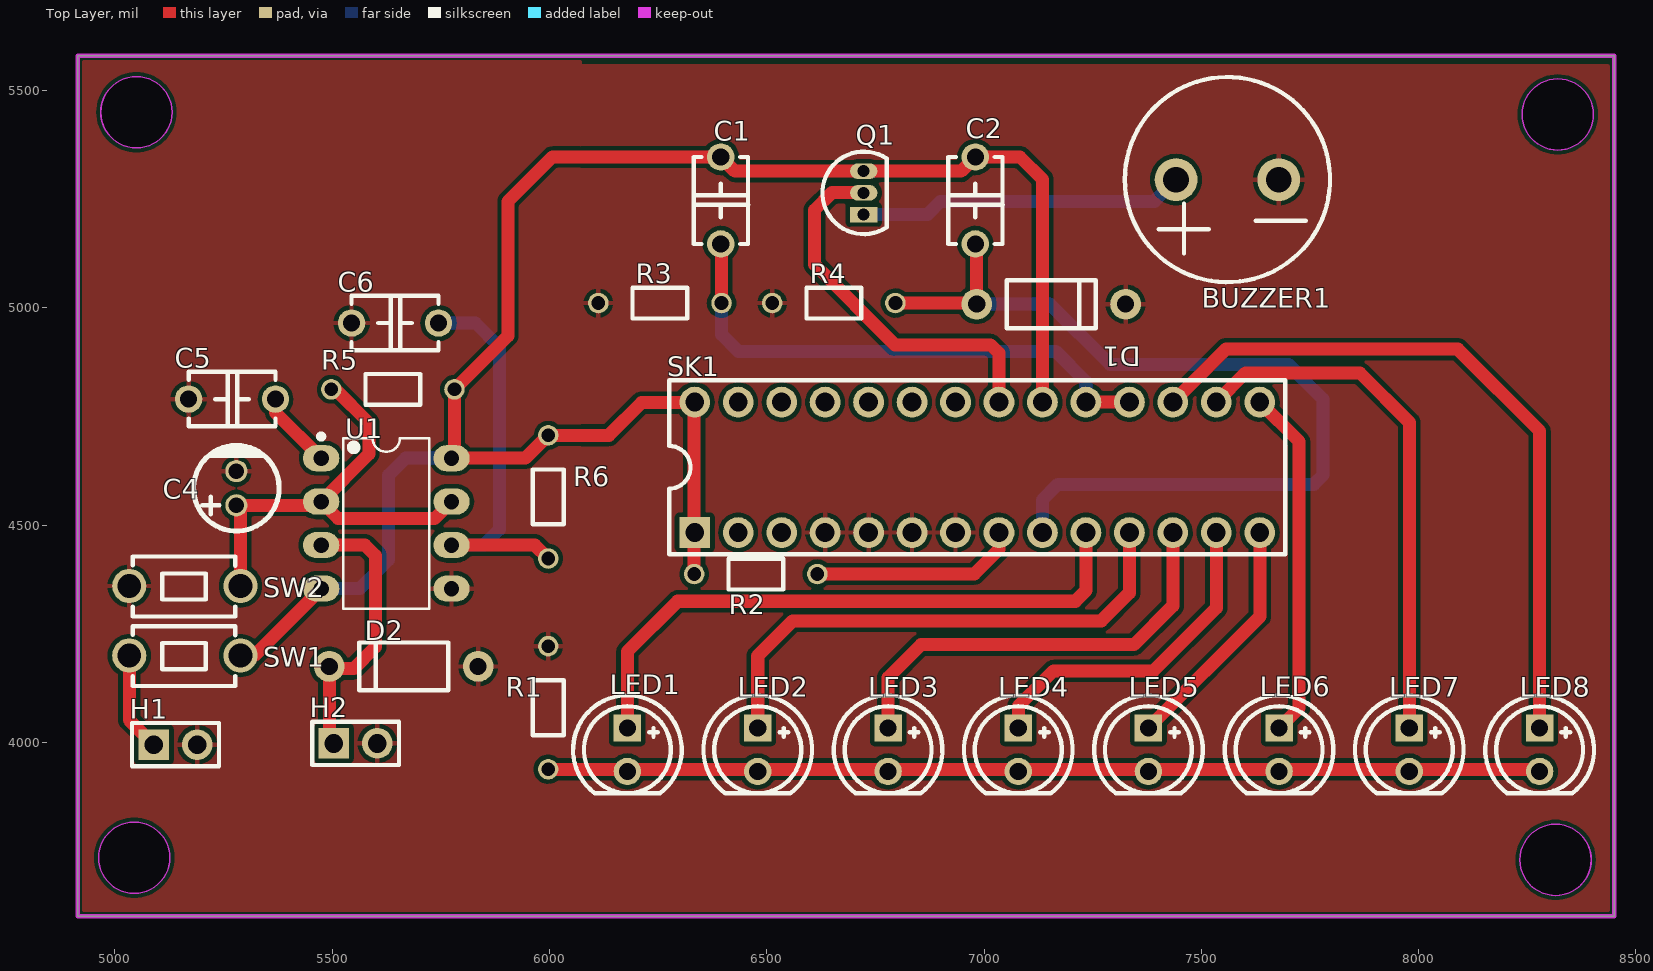
[diagram p0: Top Layer view]
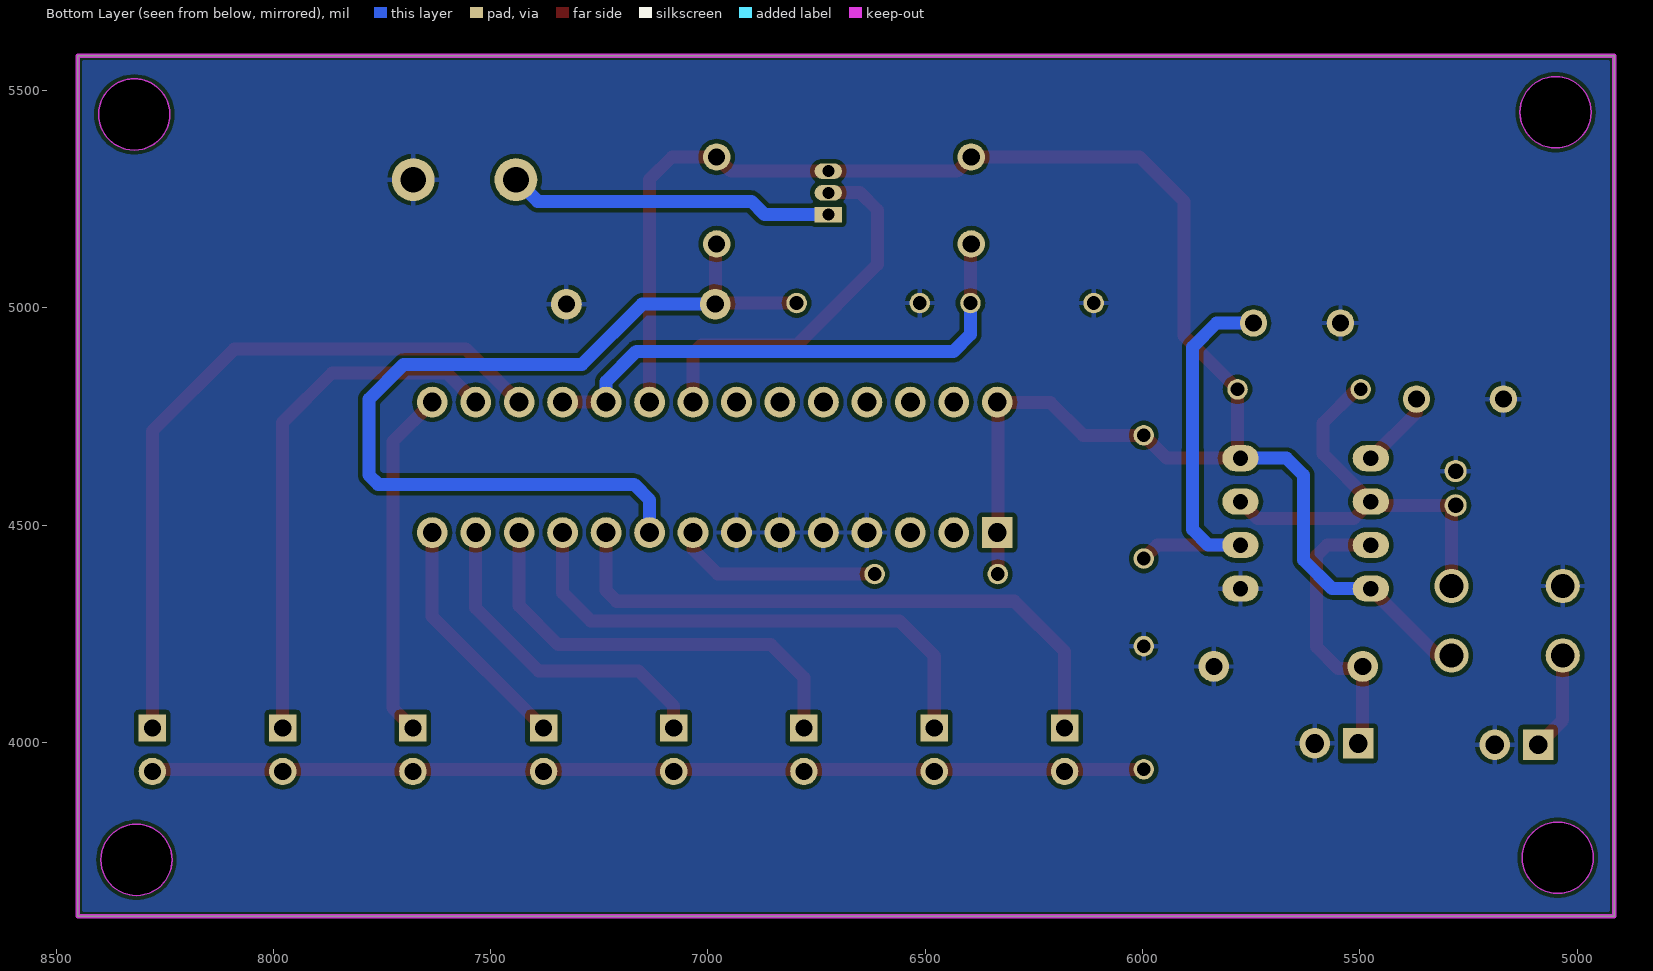
[diagram p1: Bottom Layer view, seen from below]
# Altium PCB MISC75112.pcbdoc
Units mil, origin at the board's own origin, x right, y up, seen from the top; angles counter-clockwise.
Board outline 3535 x 1980 mil, 2 copper layers (Top Layer, Bottom Layer), stack 62.206 mil thick; 29 components, 21 nets, 91 pads, 0 vias.

## Layer stack, top to bottom
Top Solder Mask Layer: solder mask 0.394, Dk 3.3
Top Layer: signal copper 1.379
Dielectric1: surface 59.449, FR4, Dk 4.5
Bottom Layer: signal copper 1.378
Bottom Solder Mask Layer: solder mask 0.394, Dk 3.3

## Board outline
4915,5580 4915,3600 8450,3600 8450,5580
cut-out: 5132.01,5450 cw(c5050,5450) 4967.99,5450 cw(c5050,5450)
cut-out: 8402.01,5445 cw(c8320,5445) 8237.99,5445 cw(c8320,5445)
cut-out: 8397.01,3730 cw(c8315,3730) 8232.99,3730 cw(c8315,3730)
cut-out: 5127.01,3735 cw(c5045,3735) 4962.99,3735 cw(c5045,3735)

## Design rules (kind name [scope] priority, off if disabled: settings)
BoardOutlineClearance copperThickness2oz_1 [All] p2 off: genericclearance=7.99 ignorepadtopadclearanceinfootprint=FALSE except(0: Arc-SplitContinuation Track-SplitContinuation SMDPad-SplitContinuation THPad-SplitContinuation Via-SplitContinuation Fill-SplitContinuation Region-SplitContinuation Poly-SplitContinuation Text-SplitContinuation Hole-SplitContinuation; 5.98: Arc-CutoutEdge SMDPad-CutoutEdge THPad-CutoutEdge Via-CutoutEdge Fill-CutoutEdge Region-CutoutEdge Text-CutoutEdge; 6.93: Hole-OutlineEdge Hole-CutoutEdge; 10: Poly-OutlineEdge Poly-CutoutEdge; 11.81: Arc-OutlineEdge Track-OutlineEdge SMDPad-OutlineEdge THPad-OutlineEdge Via-OutlineEdge Fill-OutlineEdge Region-OutlineEdge Text-OutlineEdge Track-CutoutEdge)
BoardOutlineClearance copperThickness1oz_1 [All] p4: genericclearance=4.02 ignorepadtopadclearanceinfootprint=FALSE except(0: Arc-SplitContinuation Track-SplitContinuation SMDPad-SplitContinuation THPad-SplitContinuation Via-SplitContinuation Fill-SplitContinuation Region-SplitContinuation Poly-SplitContinuation Text-SplitContinuation Hole-SplitContinuation; 6: SMDPad-CutoutEdge THPad-CutoutEdge Via-CutoutEdge Fill-CutoutEdge Region-CutoutEdge Text-CutoutEdge; 6.93: Hole-OutlineEdge Hole-CutoutEdge; 10: Poly-OutlineEdge Poly-CutoutEdge; 11.8: Arc-OutlineEdge Track-OutlineEdge SMDPad-OutlineEdge THPad-OutlineEdge Via-OutlineEdge Fill-OutlineEdge Region-OutlineEdge Text-OutlineEdge; 11.81: Arc-CutoutEdge Track-CutoutEdge)
Clearance copperThickness2oz [All] p1 off: gap=7.99 ignorepadtopadclearanceinfootprint=FALSE except(5.98: SMDPad-Track SMDPad-SMDPad THPad-Track SMDPad-THPad THPad-THPad Track-Via SMDPad-Via THPad-Via Via-Via Fill-Track Region-Track Fill-SMDPad Region-SMDPad Fill-THPad Region-THPad Fill-Via Region-Via Fill-Fill Fill-Region Region-Region Arc-Track Arc-SMDPad Arc-THPad Arc-Via Fill-Arc Region-Arc Arc-Arc Text-Track SMDPad-Text Text-THPad Text-Via Fill-Text Region-Text Arc-Text Text-Text; 6.93: Hole-Track Hole-SMDPad Hole-THPad Hole-Via Fill-Hole Region-Hole Hole-Arc Hole-Text; 10: Poly-Track Poly-SMDPad Poly-THPad Poly-Via Poly-Fill Poly-Region Poly-Poly Poly-Arc Poly-Text Poly-Hole)
Clearance copperThickness1oz [All] p3: gap=4.02 ignorepadtopadclearanceinfootprint=FALSE except(5.98: SMDPad-Track SMDPad-SMDPad THPad-Track SMDPad-THPad THPad-THPad Track-Via SMDPad-Via THPad-Via Via-Via Fill-Track Region-Track Fill-SMDPad Region-SMDPad Fill-THPad Region-THPad Fill-Via Region-Via Fill-Fill Fill-Region Region-Region; 6: Arc-Track Arc-SMDPad Arc-THPad Arc-Via Fill-Arc Region-Arc Arc-Arc Text-Track SMDPad-Text Text-THPad Text-Via Fill-Text Region-Text Arc-Text Text-Text; 6.93: Hole-Track Hole-SMDPad Hole-THPad Hole-Via Fill-Hole Region-Hole Hole-Arc Hole-Text; 10: Poly-Track Poly-SMDPad Poly-THPad Poly-Via Poly-Fill Poly-Region Poly-Poly Poly-Arc Poly-Text Poly-Hole)
Creepage creepage [All] p1: checkdistance=0 ignoreinternallayers=TRUE applytopolygonpour=TRUE
DiffPairsRouting differentialPair [All] p1: maxlimit=6 minlimit=6 mostfreqgap=6 toplayer_minwidth=5 toplayer_prefwidth=10 toplayer_maxwidth=100 toplayer_mingap=6 toplayer_prefgap=6 toplayer_maxgap=6 bottomlayer_minwidth=5 bottomlayer_prefwidth=10 bottomlayer_maxwidth=100 bottomlayer_mingap=6 bottomlayer_prefgap=6 bottomlayer_maxgap=6 maxuncoupledlength=10
HoleToHoleClearance otherClearance [All] p1: gap=11.81 allowstackedmicrovias=TRUE
Length netLength [All] p1: minlimit=0 maxlimit=0
MatchedLengths netLengthTolerance [All] p1: tolerance=1000
PasteMaskExpansion pasteMaskExpansion [All] p1: expansion=0
PlaneConnect innerPlane [All] p1: planeconnectstyle=Relief reliefexpansion=20 reliefentries=4 reliefconductorwidth=10 reliefairgap=10
PolygonConnect copperRegion [(InNet('GND'))] p1: connectstyle=Relief reliefconductorwidth=10 reliefentries=4 polygonreliefangle="90 Angle" airgapwidth=10 via.connectstyle=Relief via.reliefconductorwidth=10 via.reliefentries=4 via.polygonreliefangle="90 Angle" via.airgapwidth=10
RoutingVias viaSize [All] p1: holewidth=12.01 width=24.02 viastyle="Through Hole" minholewidth=11.81 minwidth=19.68 maxholewidth=248.03 maxwidth=393.7
SolderMaskExpansion solderMaskExpansion [IsVia] p1: expansion=-1000 istentingtop=TRUE
SolderMaskExpansion solderMaskExpansion [All] p2: expansion=2 istentingtop=FALSE
Width copperThickness2oz_2 [All] p1 off: maxlimit=100 minlimit=8 preferedwidth=10
Width copperThickness1oz_2 [All] p2: maxlimit=100 minlimit=5 preferedwidth=10

## Components (designator, comment, footprint, x,y, rotation, side; value= is the part's Value field where it differs from the comment)
BUZZER1 "buzzer" BUZ-TH_BD12.0-P6.00-D0.9-RD 7560,5295 r180 top
C1 "0.1uF" CAP-TH_L5.1-W3.2-P5.08-D0.50 6394.47,5247.04 r90 top
C2 "0.047uF" CAP-TH_L5.1-W3.2-P5.08-D0.50 6980,5247.04 r90 top
C4 "10uF" CAP-TH_BD5.0-P2.00-D0.8-FD-10UF50VC110GL 5280,4585 r90 top
C5 "10nF" CAP-TH_L5.1-W3.2-P5.08-D0.50 5270,4790 r0 top
C6 "10nF" CAP-TH_L5.1-W3.2-P5.08-D0.50 5645,4965 r0 top
D1 "" DO_1N4007 7154.47,5008.49 r180 top
D2 "" DO_1N4007 5665,4175 r0 top
H1 "" HDR-TH_2P-P2.54-V-M-1 5140,3995 r0 top
H2 "" HDR-TH_2P-P2.54-V-M-1 5554.18,3998.07 r0 top
LED1 "" LED-TH_5mm 6179.47,3983.38 r270 top
LED2 "" LED-TH_5mm 6479.47,3983.38 r270 top
LED3 "" LED-TH_5mm 6779.47,3983.38 r270 top
LED4 "" LED-TH_5mm 7078.88,3983.38 r270 top
LED5 "" LED-TH_5mm 7378.29,3983.38 r270 top
LED6 "" LED-TH_5mm 7678.99,3983.38 r270 top
LED7 "" LED-TH_5mm 7978.4,3983.38 r270 top
LED8 "" LED-TH_5mm 8278.4,3983.38 r270 top
Q1 "" S8050_TO_92 6723.29,5264.53 r90 top
R1 "1kΩ" Res_1/8W 5995,4080 r270 top
R2 "22kΩ" Res_1/8W 6475,4390 r180 top
R3 "100kΩ" Res_1/8W 6254.47,5008.49 r0 top
R4 "100kΩ" Res_1/8W 6654.47,5008.49 r0 top
R5 "10kΩ" Res_1/8W 5640,4810 r0 top
R6 "10kΩ" Res_1/8W 6000,4565 r90 top
SK1 "X5621WV-2x14-C762D1000-1000" DIP-28_L35.6-W10.2-P2.54-LS7.6-BL 6984.47,4633.07 r0 top
SW1 "" Key_TH_3.5x6x4.3 5155,4200 r0 top
SW2 "" Key_TH_3.5x6x4.3 5155,4360 r0 top
U1 "NE555" DIP-8_L9.8-W6.4-P2.54-LS7.6-BL 5624.93,4504.05 r270 top

## Footprints (in the part's own frame and the unit in brackets; to place one, negate y for a bottom-side part, rotate by r counter-clockwise, add the part's x,y. Pads: shape width x height; smd on the part's side, far side on the other; paste and mask are expansions set on the pad)
BUZ-TH_BD12.0-P6.00-D0.9-RD [mm]
  round 2.5 hole 1.5 paste+0 mask+0.05: 1(-3,0) 2(3,0)
  silkscreen extent -5.99,-5.99 5.99,5.99
CAP-TH_BD5.0-P2.00-D0.8-FD-10UF50VC110GL [mm]
  round 1.3 hole 0.9 paste+0 mask+0.051: 1(-1,0) 2(1,0)
  silkscreen extent -2.5,-2.5 2.5,2.5
CAP-TH_L5.1-W3.2-P5.08-D0.50 [mm]
  round 1.6 hole 1 paste+0 mask+0.05: 1(-2.54,0) 2(2.54,0)
  silkscreen extent -2.54,-1.6 2.54,1.59
DIP-8_L9.8-W6.4-P2.54-LS7.6-BL [mil]
  oval 60x83.66 hole 35.43 paste+0 mask+2: 1(-150,-150) 2(-50,-150) 3(50,-150) 4(150,-150) 5(150,150) 6(50,150) 7(-50,150) 8(-150,150)
  silkscreen extent -206,-156 196,99
DIP-28_L35.6-W10.2-P2.54-LS7.6-BL [mm]
  rect 1.8x1.8 hole 1.1: 1(-16.51,-3.81)
  round 1.8 hole 1.1: 2(-13.97,-3.81) 3(-11.43,-3.81) 4(-8.89,-3.81) 5(-6.35,-3.81) 6(-3.81,-3.81) 7(-1.27,-3.81) 8(1.27,-3.81) 9(3.81,-3.81) 10(6.35,-3.81) 11(8.89,-3.81) 12(11.43,-3.81) 13(13.97,-3.81) 14(16.51,-3.81) 15(16.51,3.81) 16(13.97,3.81) 17(11.43,3.81) 18(8.89,3.81) 19(6.35,3.81) 20(3.81,3.81) 21(1.27,3.81) 22(-1.27,3.81) 23(-3.81,3.81) 24(-6.35,3.81) 25(-8.89,3.81) 26(-11.43,3.81) 27(-13.97,3.81) 28(-16.51,3.81)
  silkscreen extent -18,-5.08 18,5.08
DO_1N4007 [mm]
  round 1.8 hole 1 paste+0 mask+0.051: 1(-4.35,0) 2(4.35,0)
  silkscreen extent -2.6,-1.4 2.6,1.4
HDR-TH_2P-P2.54-V-M-1 [mm]
  rect 1.8x1.8 hole 1.1: 1(-1.27,0)
  round 1.8 hole 1.1: 2(1.27,0)
  silkscreen extent -2.54,-1.27 2.54,1.27
Key_TH_3.5x6x4.3 [mil]
  round 78.7 hole 55.1 paste+0 mask+2: A(-121.44,0) B(134.46,0)
  silkscreen extent -114,-70 123,68
LED-TH_5mm [mm]
  rect 1.6x1.6 hole 1 paste+0 mask+0.051: 1(-1.27,0)
  round 1.6 hole 1 paste+0 mask+0.051: 2(1.27,0)
  silkscreen extent -3.17,-3.17 2.54,3.17
Res_1/8W [mil]
  round 47.2 hole 31.5 paste+0 mask+2: 1(-141.7,2.48) 2(141.7,2.48)
  silkscreen extent -63,-33 63,38
S8050_TO_92 [mil]
  rect 35.4x63 hole 27.6 paste+0 mask+2: 1(-50,0)
  oval 35.4x63 hole 27.6 paste+0 mask+2: 2(0,0) 3(50,0)
  silkscreen extent -95,-53 95,95

## Nets (pads, with @x,y where several pads share a name; then routed paths per layer and width w, separated by ;. In a path a pad name is that pad's centre, name@x,y a point inside that pad or via, vN(x,y) a via of type N, cw(c..) or ccw(c..) an arc to the next point about the centre after c; other vN are vias at no path point)
$1N42: LED1.1 SK1.10 | length 1422.7
  Top Layer w30: LED1.1 6179.47,4209.47 6295,4325 7210,4325 7234.47,4349.47 SK1.10
$1N43: LED2.1 SK1.11 | length 1219.7
  Top Layer w30: LED2.1 6479.47,4199.47 6560,4280 7270,4280 7334.47,4344.47 SK1.11
$1N44: LED3.1 SK1.12 | length 1008
  Top Layer w30: LED3.1 6779.47,4149.47 6855,4225 7345,4225 7434.47,4314.47 SK1.12
$1N45: LED4.1 SK1.13 | length 773.1
  Top Layer w30: LED4.1 7078.88,4083.88 7160,4165 7390,4165 7534.47,4309.47 SK1.13
$1N46: LED5.1 SK1.14 | length 555.8
  Top Layer w30: LED5.1 7634.47,4289.56 SK1.14
$1N47: LED6.1 SK1.15 | length 806.2
  Top Layer w30: SK1.15 7725,4692.53 7725,4079.4 LED6.1
$1N48: LED7.1 SK1.16 | length 1221.8
  Top Layer w30: SK1.16 7601.4,4850 7865,4850 7978.4,4736.6 LED7.1
$1N49: LED8.1 SK1.17 | length 1655.7
  Top Layer w30: SK1.17 7556.4,4905 8090,4905 8278.4,4716.6 LED8.1
$1N50: LED1.2 LED2.2 LED3.2 LED4.2 LED5.2 LED6.2 LED7.2 LED8.2 R1.2 | length 2283
  Top Layer w30: R1.2 8273.48,3938.3 LED8.2
$1N52: C1.2 C2.2 Q1.3 R2.2 R5.2 R6.2 SK1.1 SK1.20 SK1.28 SW1.B U1.4 U1.8 | length 4272.4
  Top Layer w30: SW1.B 5320.88,4200 U1.4 ; R2.2 SK1.28@6333.3,4781.9 ; SK1.28 SK1.28@6333.3,4781.9 ; SK1.20 7134.47,5295.53 7082.96,5347.04 C2.2 6947.49,5314.53 Q1.3 6426.97,5314.53 C1.2 6007.04,5347.04 5905,5245 5905,4935.78 R5.2 5781.7,4660.82 U1.8 5944.88,4654.05 R6.2 6136.7,4706.7 6211.9,4781.9 SK1.28@6333.3,4781.9
  Bottom Layer w30: U1.4 5564.05,4354.05 5630,4420 5630,4615 5669.05,4654.05 U1.8
$1N53: R2.1 SK1.8 | length 480
  Top Layer w30: R2.1 6977.52,4387.52 7034.47,4444.47 SK1.8
$1N54: C1.1 R3.2 SK1.18 SK1.19 | length 1239.5
  Top Layer w30: C1.1 6396.17,5145.34 R3.2 ; SK1.19 SK1.18
  Bottom Layer w30: R3.2 6396.17,4938.83 6435,4900 7165,4900 7234.47,4830.53 SK1.19
$1N56: C2.1 D1.2 R4.2 SK1.9 | length 2134.5
  Top Layer w30: R4.2 6980.73,5010.97 D1.2 6983.21,5143.83 C2.1
  Bottom Layer w30: D1.2 7151.51,5008.49 7290,4870 7700,4870 7780,4790 7780,4615 7758.79,4593.79 7170,4593.79 7134.47,4558.25 SK1.9
$1N59: Q1.2 SK1.21 | length 876.7
  Top Layer w30: Q1.2 6722.82,5265 6650,5265 6610,5225 6610,5100 6795,4915 7015,4915 7034.47,4895.53 SK1.21
$1N61: BUZZER1.2 Q1.1 | length 751.9
  Bottom Layer w30: Q1.1 6869.53,5214.53 6900,5245 7391.89,5245 BUZZER1.2
$1N63: C4.1 R5.1 SW2.B U1.2 U1.7 | length 1065.4
  Top Layer w30: SW2.B 5289.46,4536.17 C4.1 5466.51,4545.63 U1.2 ; R5.1 5507.52,4812.48 5585,4735 5585,4664.12 U1.2 ; U1.7 5736.14,4515.26 5513.72,4515.26 U1.2
$1N64: C6.2 R6.1 U1.6 | length 943.1
  Top Layer w30: U1.6 5966.77,4454.05 R6.1
  Bottom Layer w30: C6.2 5830,4965 5885,4910 5885,4490 5849.05,4454.05 U1.6
$1N66: H1.1 SW1.A | length 228.4
  Top Layer w30: SW1.A 5033.56,4051.44 H1.1
$1N71: C5.2 U1.1 | length 179.4
  Top Layer w30: C5.2 5370,4758.98 U1.1
$1N73: D2.1 H2.1 U1.3 | length 655.3
  Top Layer w30: U1.3 5575.95,4454.05 5600,4430 5600,4220 5550,4170 5498.74,4170 D2.1 5493.74,4008.51 H2.1
GND: BUZZER1.1 C4.2 C5.1 C6.1 D1.1 D2.2 H1.2 H2.2 R1.1 R3.1 R4.1 SK1.4 SK1.5 SK1.6 SK1.7 SW2.A U1.5
pads on no net: SK1.2 SK1.3 SK1.22 SK1.23 SK1.24 SK1.25 SK1.26 SK1.27

## Polygon pours and split planes (outlines as drawn)
GND on Top Layer (solid, remove dead copper, pour order 0): 3000,7155 3000,4605 6075,4605 6075,7155
GND on Bottom Layer (solid, remove dead copper, pour order 4): 3140,7115 3140,4675 5925,4675 5925,7115
GND on Top Layer (solid, remove dead copper, pour order 2): 4740,5560 4740,3005 9155,3005 9155,5560
GND on Bottom Layer (solid, remove dead copper, pour order 6): 4605,5615 4605,3000 8995,3000 8995,5615

## Keep-outs
Board Outline Layer:
  region: 5132.01,5450 cw(c5050,5450) 4967.99,5450 cw(c5050,5450)
  circle w0.1: c5050,5450 r82.01
  region: 5132.01,5450 5131.61,5441.96 5130.43,5434 5128.47,5426.19 5125.76,5418.62 5122.32,5411.34 5118.19,5404.44 5113.39,5397.98 5107.99,5392.01 5102.02,5386.61 5095.56,5381.81 5088.66,5377.68 5081.38,5374.24 5073.81,5371.53 5066,5369.57 5058.04,5368.39 5050,5367.99 5041.96,5368.39 5034,5369.57 5026.19,5371.53 5018.62,5374.24 5011.34,5377.68 5004.44,5381.81 4997.98,5386.61 4992.01,5392.01 4986.61,5397.98 4981.81,5404.44 4977.68,5411.34 4974.24,5418.62 4971.53,5426.19 4969.57,5434 4968.39,5441.96 4967.99,5450 4968.39,5458.04 4969.57,5466 4971.53,5473.81 4974.24,5481.38 4977.68,5488.66 4981.81,5495.56 4986.61,5502.02 4992.01,5507.99 4997.98,5513.39 5004.44,5518.19 5011.34,5522.32 5018.62,5525.76 5026.19,5528.47 5034,5530.43 5041.96,5531.61 5050,5532.01 5058.04,5531.61 5066,5530.43 5073.81,5528.47 5081.38,5525.76 5088.66,5522.32 5095.56,5518.19 5102.02,5513.39 5107.99,5507.99 5113.39,5502.02 5118.19,5495.56 5122.32,5488.66 5125.76,5481.38 5128.47,5473.81 5130.43,5466 5131.61,5458.04
  region: 8402.01,5445 cw(c8320,5445) 8237.99,5445 cw(c8320,5445)
  circle w0.1: c8320,5445 r82.01
  region: 8402.01,5445 8401.61,5436.96 8400.43,5429 8398.47,5421.19 8395.76,5413.62 8392.32,5406.34 8388.19,5399.44 8383.39,5392.98 8377.99,5387.01 8372.02,5381.61 8365.56,5376.81 8358.66,5372.68 8351.38,5369.24 8343.81,5366.53 8336,5364.57 8328.04,5363.39 8320,5362.99 8311.96,5363.39 8304,5364.57 8296.19,5366.53 8288.62,5369.24 8281.34,5372.68 8274.44,5376.81 8267.98,5381.61 8262.01,5387.01 8256.61,5392.98 8251.81,5399.44 8247.68,5406.34 8244.24,5413.62 8241.53,5421.19 8239.57,5429 8238.39,5436.96 8237.99,5445 8238.39,5453.04 8239.57,5461 8241.53,5468.81 8244.24,5476.38 8247.68,5483.66 8251.81,5490.56 8256.61,5497.02 8262.01,5502.99 8267.98,5508.39 8274.44,5513.19 8281.34,5517.32 8288.62,5520.76 8296.19,5523.47 8304,5525.43 8311.96,5526.61 8320,5527.01 8328.04,5526.61 8336,5525.43 8343.81,5523.47 8351.38,5520.76 8358.66,5517.32 8365.56,5513.19 8372.02,5508.39 8377.99,5502.99 8383.39,5497.02 8388.19,5490.56 8392.32,5483.66 8395.76,5476.38 8398.47,5468.81 8400.43,5461 8401.61,5453.04
  region: 8397.01,3730 cw(c8315,3730) 8232.99,3730 cw(c8315,3730)
  circle w0.1: c8315,3730 r82.01
  region: 8397.01,3730 8396.61,3721.96 8395.43,3714 8393.47,3706.19 8390.76,3698.62 8387.32,3691.34 8383.19,3684.44 8378.39,3677.98 8372.99,3672.01 8367.02,3666.61 8360.56,3661.81 8353.66,3657.68 8346.38,3654.24 8338.81,3651.53 8331,3649.57 8323.04,3648.39 8315,3647.99 8306.96,3648.39 8299,3649.57 8291.19,3651.53 8283.62,3654.24 8276.34,3657.68 8269.44,3661.81 8262.98,3666.61 8257.01,3672.01 8251.61,3677.98 8246.81,3684.44 8242.68,3691.34 8239.24,3698.62 8236.53,3706.19 8234.57,3714 8233.39,3721.96 8232.99,3730 8233.39,3738.04 8234.57,3746 8236.53,3753.81 8239.24,3761.38 8242.68,3768.66 8246.81,3775.56 8251.61,3782.02 8257.01,3787.99 8262.98,3793.39 8269.44,3798.19 8276.34,3802.32 8283.62,3805.76 8291.19,3808.47 8299,3810.43 8306.96,3811.61 8315,3812.01 8323.04,3811.61 8331,3810.43 8338.81,3808.47 8346.38,3805.76 8353.66,3802.32 8360.56,3798.19 8367.02,3793.39 8372.99,3787.99 8378.39,3782.02 8383.19,3775.56 8387.32,3768.66 8390.76,3761.38 8393.47,3753.81 8395.43,3746 8396.61,3738.04
  region: 5127.01,3735 cw(c5045,3735) 4962.99,3735 cw(c5045,3735)
  circle w0.1: c5045,3735 r82.01
  region: 5127.01,3735 5126.61,3726.96 5125.43,3719 5123.47,3711.19 5120.76,3703.62 5117.32,3696.34 5113.19,3689.44 5108.39,3682.98 5102.99,3677.01 5097.02,3671.61 5090.56,3666.81 5083.66,3662.68 5076.38,3659.24 5068.81,3656.53 5061,3654.57 5053.04,3653.39 5045,3652.99 5036.96,3653.39 5029,3654.57 5021.19,3656.53 5013.62,3659.24 5006.34,3662.68 4999.44,3666.81 4992.98,3671.61 4987.01,3677.01 4981.61,3682.98 4976.81,3689.44 4972.68,3696.34 4969.24,3703.62 4966.53,3711.19 4964.57,3719 4963.39,3726.96 4962.99,3735 4963.39,3743.04 4964.57,3751 4966.53,3758.81 4969.24,3766.38 4972.68,3773.66 4976.81,3780.56 4981.61,3787.02 4987.01,3792.99 4992.98,3798.39 4999.44,3803.19 5006.34,3807.32 5013.62,3810.76 5021.19,3813.47 5029,3815.43 5036.96,3816.61 5045,3817.01 5053.04,3816.61 5061,3815.43 5068.81,3813.47 5076.38,3810.76 5083.66,3807.32 5090.56,3803.19 5097.02,3798.39 5102.99,3792.99 5108.39,3787.02 5113.19,3780.56 5117.32,3773.66 5120.76,3766.38 5123.47,3758.81 5125.43,3751 5126.61,3743.04
  lines w10: 4915,3600 4915,5580 8450,5580 8450,3600 4915,3600

## Silkscreen, mask and mechanical layers (free items; w line width, h text height)
Mechanical Layer:
  circle w0.1: c5050,5450 r82.01
  circle w0.1: c8320,5445 r82.01
  circle w0.1: c8315,3730 r82.01
  circle w0.1: c5045,3735 r82.01